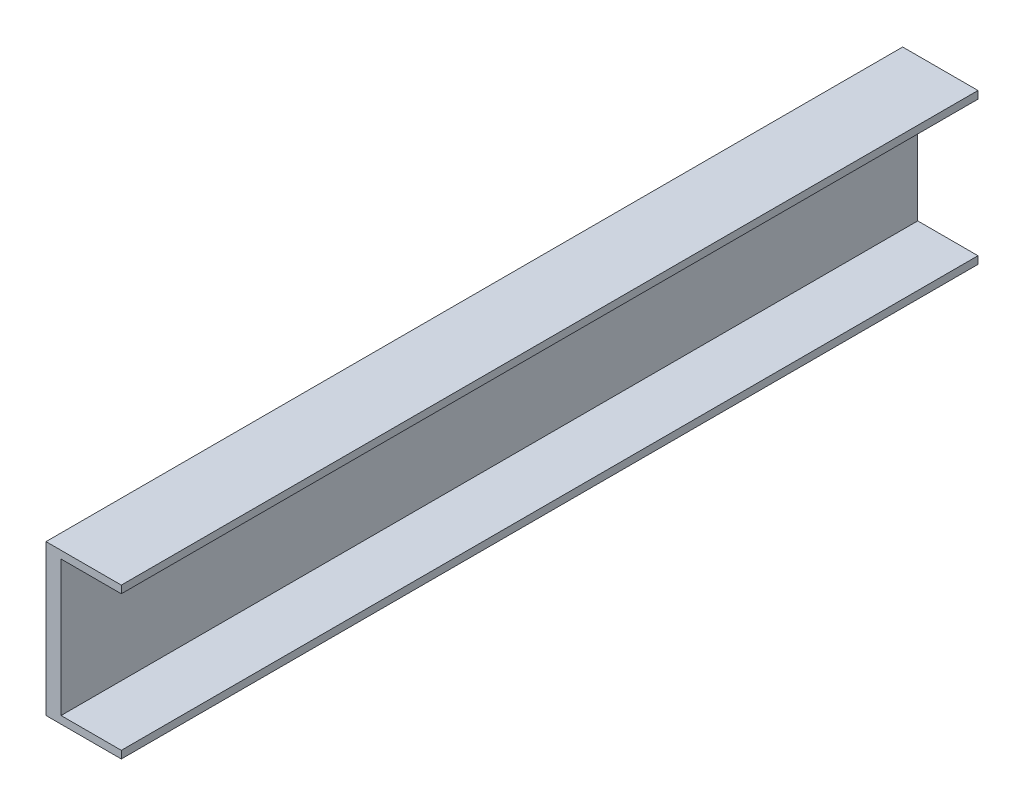
SolidWorks part; units mm, degrees
ref_plane "Front Plane" through (0, 0, 0) normal (0, 0, 1) x (1, 0, 0)
ref_plane "Top Plane" through (0, 0, 0) normal (0, 1, 0) x (1, 0, 0)
ref_plane "Right Plane" through (0, 0, 0) normal (1, 0, 0) x (0, 0, -1)
sketch "Sketch1" plane through (0, 0, 0) normal (0, 0, 1) x (1, 0, 0)
  line L0 (0, 0) -> (-40, 0)
  line L1 (-40, 0) -> (-40, 80)
  line L2 (-40, 80) -> (0, 80)
  line L3 (0, 80) -> (0, 76)
  line L4 (0, 76) -> (-32, 76)
  line L5 (-32, 76) -> (-32, 4)
  line L6 (-32, 4) -> (0, 4)
  line L7 (0, 4) -> (0, 0)
  dimension "D1" = 80
  dimension "D2" = 40
  dimension "D3" = 40
  dimension "D4" = 4
  dimension "D5" = 4
  dimension "D6" = 8
sheet metal parameters "Sheet metal 1" thickness 3 parameters "D1"=3
extrude "Extrude1" add sketch "Sketch1" along normal blind 455
